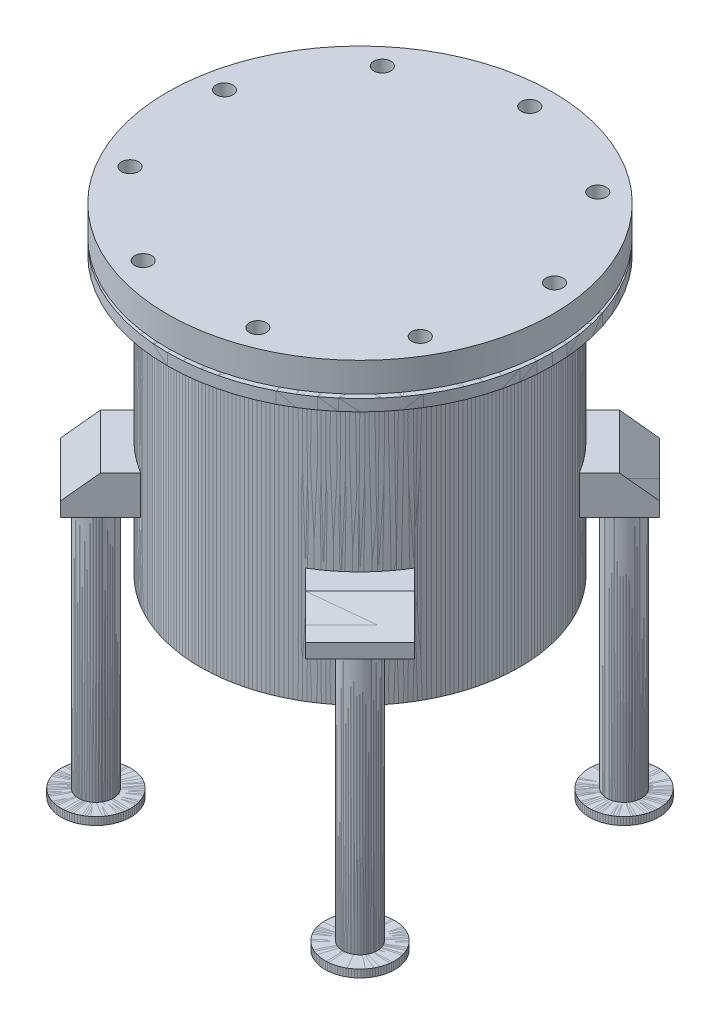
from build123d import *

# Parameters (mm, degrees)
SKETCH1_R               = 415
BOSS_EXTRUDE1_DEPTH     = 750
SHELL1_T                = -15
BOSS_EXTRUDE2_START     = -30
SKETCH2_R               = 500
SKETCH2_R_2             = 415
BOSS_EXTRUDE2_DEPTH     = 30
SKETCH3_R               = 500
BOSS_EXTRUDE3_DEPTH     = 86
CUT_EXTRUDE1_DEPTH      = 1095.941094306
CUT_EXTRUDE1_DEPTH_BACK = 1095.941094306
SKETCH4_W               = 1053.25185681
SKETCH4_H               = 10
BOSS_EXTRUDE4_START     = 100
BOSS_EXTRUDE4_DEPTH     = 100
CUT_EXTRUDE2_DEPTH      = 1163.031564217
CUT_EXTRUDE2_DEPTH_BACK = 1163.031564217
SKETCH7_R               = 45
BOSS_EXTRUDE5_DEPTH     = 700
SKETCH8_R               = 90.375990814
BOSS_EXTRUDE6_DEPTH     = 20
SKETCH9_R               = 22.185346079
CUT_EXTRUDE3_DEPTH      = 136
CIRPATTERN1_COUNT       = 9
CIRPATTERN5_COUNT       = 4
SKETCH10_R              = 15
CUT_EXTRUDE4_DEPTH      = 722


with BuildPart() as part:
    # Sketch1 → Boss-Extrude1 (new body)
    with BuildSketch(Plane(origin=(0, 0, 0), x_dir=(1, 0, 0), z_dir=(0, 1, 0))):
        with Locations(Location((0, 0, 0), (0, 0, 270))):
            Circle(SKETCH1_R)
    extrude(amount=BOSS_EXTRUDE1_DEPTH)

    # Shell1
    shell1_openings = [part.faces().sort_by_distance(p)[0] for p in [
        (0, 750, 0),
    ]]
    offset(amount=SHELL1_T, openings=shell1_openings, kind=Kind.INTERSECTION)

    # Sketch2 → Boss-Extrude2 (add)
    with BuildSketch(Plane(origin=(0, 750, 0), x_dir=(1, 0, 0), z_dir=(0, 1, 0)).offset(BOSS_EXTRUDE2_START)):
        with Locations(Location((0, 0, 0), (0, 0, 270))):
            Circle(SKETCH2_R)
        with Locations(Location((0, 0, 0), (0, 0, 270))):
            Circle(SKETCH2_R_2, mode=Mode.SUBTRACT)
    extrude(amount=BOSS_EXTRUDE2_DEPTH)

    # Sketch5 → Boss-Extrude4 (add)
    with BuildSketch(Plane(origin=(0, 300, 0), x_dir=(-1, 0, 0), z_dir=(0, -1, 0)).offset(BOSS_EXTRUDE4_START)):
        with BuildLine():
            Line((355.513241309, -214.091885072), (459.619407771, -318.198051534))
            Line((459.619407771, -318.198051534), (318.198051534, -459.619407771))
            Line((318.198051534, -459.619407771), (214.091885072, -355.513241309))
            ThreePointArc((214.091885072, -355.513241309), (293.449314192, -293.449314192), (355.513241309, -214.091885072))
        make_face()
        with BuildLine():
            Line((-459.619407771, 318.198051534), (-355.513241309, 214.091885072))
            ThreePointArc((-355.513241309, 214.091885072), (-293.449314192, 293.449314192), (-214.091885072, 355.513241309))
            Line((-214.091885072, 355.513241309), (-318.198051534, 459.619407771))
            Line((-318.198051534, 459.619407771), (-459.619407771, 318.198051534))
        make_face()
    extrude(amount=-BOSS_EXTRUDE4_DEPTH)

    # Sketch6 → Cut-Extrude2 (cut, two sides: drawn at the far end of the back side and taken through both)
    with BuildSketch(Plane(origin=(70.710678119, 0, 70.710678119), x_dir=(0.7071067811865488, 0, -0.7071067811865462), z_dir=(0.7071067811865462, 0, 0.7071067811865488)).offset(-CUT_EXTRUDE2_DEPTH_BACK)):
        Polygon((-550, 300), (-550, 237.083154956), (-476.385823731, 300), align=None)
        Polygon((550, 237.083154956), (476.385823731, 300), (550, 300), align=None)
    extrude(amount=CUT_EXTRUDE2_DEPTH + CUT_EXTRUDE2_DEPTH_BACK, mode=Mode.SUBTRACT)

    # Sketch7 → Boss-Extrude5 (add)
    with BuildSketch(Plane.XZ.offset(-200)):
        with Locations(Location((-342.946788875, 342.946788875, 0), (0, 0, 270))):
            Circle(SKETCH7_R)
        with Locations(Location((342.946788875, -342.946788875, 0), (0, 0, 90))):
            Circle(SKETCH7_R)
    extrude(amount=BOSS_EXTRUDE5_DEPTH)

    # Sketch8 → Boss-Extrude6 (add)
    with BuildSketch(Plane.XZ.offset(500)):
        with Locations(Location((-342.946788875, 342.946788875, 0), (0, 0, 270))):
            Circle(SKETCH8_R)
        with Locations(Location((342.946788875, -342.946788875, 0), (0, 0, 270))):
            Circle(SKETCH8_R)
    extrude(amount=-BOSS_EXTRUDE6_DEPTH)


with BuildPart() as body_2:
    # Sketch3 → Boss-Extrude3 (new body)
    with BuildSketch(Plane(origin=(0, 750, 0), x_dir=(1, 0, 0), z_dir=(0, 1, 0))):
        with Locations(Location((0, 0, 0), (0, 0, 270))):
            Circle(SKETCH3_R)
    extrude(amount=BOSS_EXTRUDE3_DEPTH)

    # Sketch4 → Cut-Extrude1 (cut, two sides: drawn at the far end of the back side and taken through both)
    with BuildSketch(Plane.XY.offset(-CUT_EXTRUDE1_DEPTH_BACK)):
        with Locations((26.625928405, 755)):
            Rectangle(SKETCH4_W, SKETCH4_H)
    extrude(amount=CUT_EXTRUDE1_DEPTH + CUT_EXTRUDE1_DEPTH_BACK, mode=Mode.SUBTRACT)


with BuildPart() as cut_extrude3_tool:
    # Sketch9 → Cut-Extrude3 (new body)
    with BuildSketch(Plane(origin=(0, 836, 0), x_dir=(1, 0, 0), z_dir=(0, 1, 0))):
        with Locations(Location((2.802795327, 438.062339014, 0), (0, 0, 270))):
            Circle(SKETCH9_R)
    cut_extrude3 = extrude(amount=-CUT_EXTRUDE3_DEPTH)


with BuildPart() as part_1:
    add(part.part)

    # Cut-Extrude3: cut by cut_extrude3_tool
    add(cut_extrude3_tool.part, mode=Mode.SUBTRACT)


with BuildPart() as body_2_1:
    add(body_2.part)

    # Cut-Extrude3: cut by cut_extrude3_tool
    add(cut_extrude3_tool.part, mode=Mode.SUBTRACT)


with BuildPart() as cirpattern1_tool:
    # CirPattern1: Cut-Extrude3 ×9 about axis
    cirpattern1_axis = Axis((0, 0, 0), (0, 1, 0))
    for i in range(1, CIRPATTERN1_COUNT):
        add(cut_extrude3.rotate(cirpattern1_axis, i * 360 / CIRPATTERN1_COUNT))


with BuildPart() as part_2:
    add(part_1.part)

    # CirPattern1: cut by cirpattern1_tool
    add(cirpattern1_tool.part, mode=Mode.SUBTRACT)


with BuildPart() as body_2_2:
    add(body_2_1.part)

    # CirPattern1: cut by cirpattern1_tool
    add(cirpattern1_tool.part, mode=Mode.SUBTRACT)


with BuildPart() as cirpattern5_1:
    # CirPattern5: pattern copy
    add(part_2.part.rotate(Axis((0, 0, 0), (0, 1, 0)), 1 * 360 / CIRPATTERN5_COUNT))


with BuildPart() as cirpattern5_2:
    # CirPattern5: pattern copy
    add(part_2.part.rotate(Axis((0, 0, 0), (0, 1, 0)), 2 * 360 / CIRPATTERN5_COUNT))


with BuildPart() as cirpattern5_3:
    # CirPattern5: pattern copy
    add(part_2.part.rotate(Axis((0, 0, 0), (0, 1, 0)), 3 * 360 / CIRPATTERN5_COUNT))


with BuildPart() as cut_extrude4_tool:
    # Sketch10 → Cut-Extrude4 (new body)
    with BuildSketch(Plane(origin=(0, 0, 0), x_dir=(0, 0, -1), z_dir=(1, 0, 0))):
        with Locations((0, 500)):
            Circle(SKETCH10_R)
    extrude(amount=-CUT_EXTRUDE4_DEPTH)


with BuildPart() as part_3:
    add(part_2.part)

    # Cut-Extrude4: cut by cut_extrude4_tool
    add(cut_extrude4_tool.part, mode=Mode.SUBTRACT)


with BuildPart() as cirpattern5_1_1:
    add(cirpattern5_1.part)

    # Cut-Extrude4: cut by cut_extrude4_tool
    add(cut_extrude4_tool.part, mode=Mode.SUBTRACT)


with BuildPart() as cirpattern5_2_1:
    add(cirpattern5_2.part)

    # Cut-Extrude4: cut by cut_extrude4_tool
    add(cut_extrude4_tool.part, mode=Mode.SUBTRACT)


with BuildPart() as cirpattern5_3_1:
    add(cirpattern5_3.part)

    # Cut-Extrude4: cut by cut_extrude4_tool
    add(cut_extrude4_tool.part, mode=Mode.SUBTRACT)


solid = Compound([body_2_2.part, part_3.part, cirpattern5_1_1.part, cirpattern5_2_1.part, cirpattern5_3_1.part])
